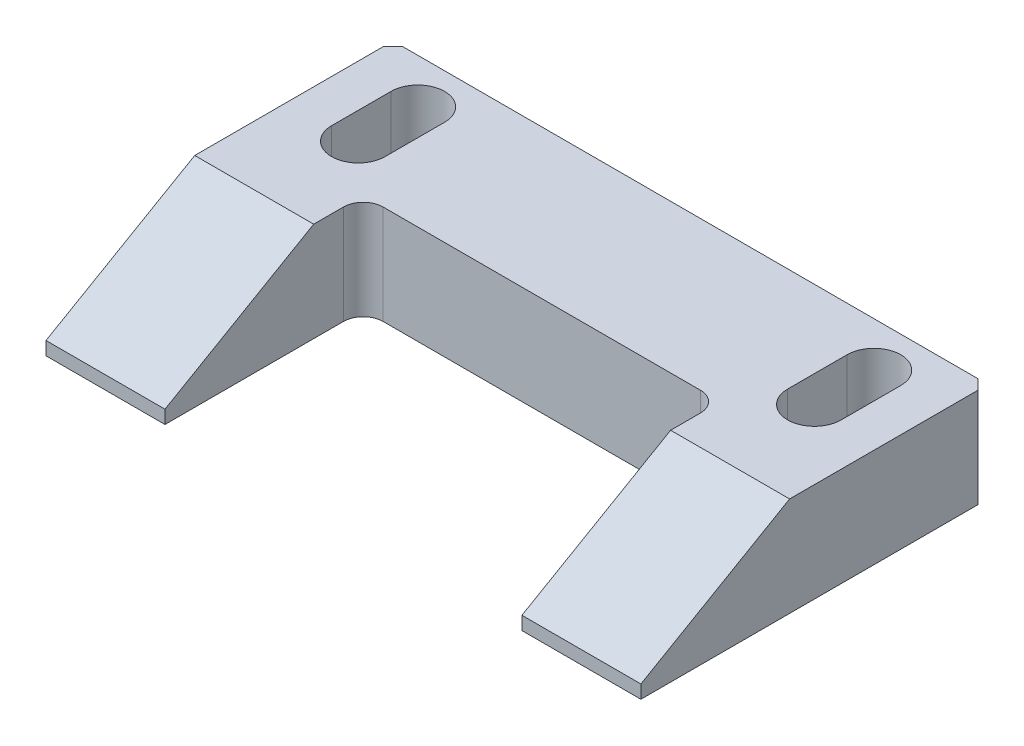
SolidWorks part; units mm, degrees
ref_plane "Front Plane" through (0, 0, 0) normal (0, 0, 1) x (1, 0, 0)
ref_plane "Top Plane" through (0, 0, 0) normal (0, 1, 0) x (1, 0, 0)
ref_plane "Right Plane" through (0, 0, 0) normal (1, 0, 0) x (0, 0, -1)
sketch "Sketch1" plane through (0, 0, 0) normal (0, 1, 0) x (1, 0, 0)
  line L1 (-30, 17.5) -> (30, 17.5)
  line L2 (-30, 17.5) -> (-30, -17.5)
  line L3 (-30, -17.5) -> (30, -17.5)
  line L4 (30, 17.5) -> (30, -17.5)
  line L5 (-30, 17.5) -> (30, -17.5) construction
  line L6 (-30, -17.5) -> (30, 17.5) construction
  point P0 (0, 0)
  dimension "D1" = 60
  dimension "D2" = 35
extrude "Boss-Extrude1" add sketch "Sketch1" along normal blind 10
chamfer "Chamfer1" distance 15 angle 30 1 edges at (0, 10, 17.5)
sketch "Sketch2" plane through (0, 10, 0) normal (0, 1, 0) x (1, 0, 0)
  line L0 (30, -17.5) -> (-30, -17.5) construction
  line L1 (-18, -17.5) -> (18, -17.5)
  line L2 (-18, -17.5) -> (-18, 2.5)
  line L3 (-18, 2.5) -> (18, 2.5)
  line L4 (18, -17.5) -> (18, 2.5)
  line L5 (0, 17.5) -> (0, 2.5) construction
  line L6 (30, 17.5) -> (-30, 17.5) construction
  line L7 (-30, -17.5) -> (-30, -2.5) construction
  dimension "D1" = 12
  dimension "D2" = 15
extrude "Cut-Extrude1" cut sketch "Sketch2" against normal through all
fillet "Fillet1" radius 2 2 edges at (18, 5, -2.5) (-18, 5, -2.5)
sketch "Sketch3" plane through (0, 10, 0) normal (0, 1, 0) x (1, 0, 0)
  line L0 (-23, 13) -> (-23, 7) construction
  line L1 (-20.3, 13) -> (-20.3, 7)
  line L2 (-25.7, 13) -> (-25.7, 7)
  line L3 (30, 17.5) -> (-30, 17.5) construction
  arc A0 (-20.3, 13) -> (-25.7, 13) centre (-23, 13) ccw
  arc A1 (-25.7, 7) -> (-20.3, 7) centre (-23, 7) ccw
  point P2 (-23, 10)
  dimension "D1" = 5.4
  dimension "D2" = 6
  dimension "D3" = 7.5
  dimension "D4" = 23
extrude "Cut-Extrude2" cut sketch "Sketch3" against normal through all
mirror "Mirror1" about plane through (0, 0, 0) normal (1, 0, 0) of "Cut-Extrude2"
chamfer "Chamfer2" distance 1 angle 45 2 edges at (30, 5, -17.5) (-30, 5, -17.5)
